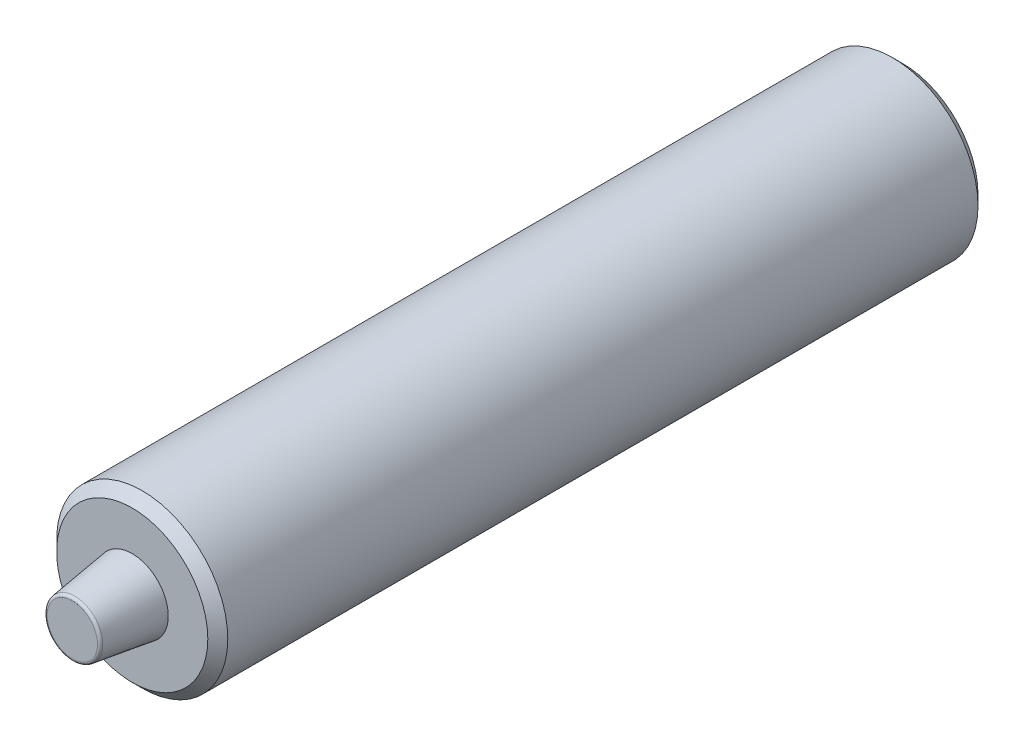
from build123d import *

# Parameters (mm, degrees)
CUT_EXTRUDE1_DEPTH = 5
SKETCH5_W          = 12
SKETCH5_H          = 4
CUT_EXTRUDE2_DEPTH = 3


with BuildPart() as part:
    # Sketch1 → Revolve1 (revolve)
    with BuildSketch(Plane(origin=(0, 0, 0), x_dir=(0, 0, -1), z_dir=(1, 0, 0)), mode=Mode.PRIVATE) as revolve1_sk:
        Polygon((0, 0), (0, 5.3), (0.7, 6), (53.3, 6), (54, 5.3), (54, 0), align=None)
    revolve(revolve1_sk.sketch.rotate(Axis((0, 0, -54), (0, 0, 1)), 270), axis=Axis((0, 0, -54), (0, 0, 1)))

    # Sketch2 → Cut-Revolve1 (revolve, cut)
    with BuildSketch(Plane(origin=(0, 0, 0), x_dir=(0, 0, -1), z_dir=(1, 0, 0)), mode=Mode.PRIVATE) as cut_revolve1_sk:
        Polygon((37, 0), (37, 3.4585), (49, 3.4585), (49, 4), (53.2, 4), (54, 4.8), (54, 0), align=None)
    revolve(cut_revolve1_sk.sketch.rotate(Axis((0, 0, -54), (0, 0, 1)), 270), axis=Axis((0, 0, -54), (0, 0, 1)), mode=Mode.SUBTRACT)

    # Sketch3 → Revolve2 (revolve)
    with BuildSketch(Plane(origin=(0, 0, 0), x_dir=(0, 0, -1), z_dir=(1, 0, 0)), mode=Mode.PRIVATE) as revolve2_sk:
        with BuildLine():
            Line((-4.2, 0), (-4.2, 1.762627227))
            ThreePointArc((-4.2, 1.762627227), (-4.150941916, 1.893839033), (-4.02783462, 1.960680841))
            Line((-4.02783462, 1.960680841), (2.3, 2.85))
            Line((2.3, 2.85), (2.3, 0))
            Line((2.3, 0), (-4.2, 0))
        make_face()
    revolve(revolve2_sk.sketch.rotate(Axis((0, 0, -2.3), (0, 0, 1)), 90), axis=Axis((0, 0, -2.3), (0, 0, 1)))

    # Sketch4 → Cut-Extrude1 (cut)
    with BuildSketch(Plane.XY.offset(-54)):
        Polygon((-4, -2.309401077), (0, -4.618802154), (4, -2.309401077), (4, 2.309401077), (0, 4.618802154), (-4, 2.309401077), align=None)
    extrude(amount=CUT_EXTRUDE1_DEPTH, mode=Mode.SUBTRACT)

    # Sketch5 → Revolve3 (revolve)
    with BuildSketch(Plane(origin=(0, 0, 0), x_dir=(0, 0, -1), z_dir=(1, 0, 0)), mode=Mode.PRIVATE) as revolve3_sk:
        with Locations((39, 2)):
            Rectangle(SKETCH5_W, SKETCH5_H)
    revolve(revolve3_sk.sketch.rotate(Axis((0, 0, -45), (0, 0, 1)), 270), axis=Axis((0, 0, -45), (0, 0, 1)))

    # Sketch6 → Cut-Extrude2 (cut)
    with BuildSketch(Plane.XY.offset(-45)):
        Polygon((-2, -1.154700538), (0, -2.309401077), (2, -1.154700538), (2, 1.154700538), (0, 2.309401077), (-2, 1.154700538), align=None)
    extrude(amount=CUT_EXTRUDE2_DEPTH, mode=Mode.SUBTRACT)

    # Sketch7 → Cut-Revolve2 (revolve, cut)
    with BuildSketch(Plane(origin=(0, 0, 0), x_dir=(0, 0, -1), z_dir=(1, 0, 0)), mode=Mode.PRIVATE) as cut_revolve2_sk:
        Polygon((40.845299462, 0), (42, 2), (42, 0), align=None)
    revolve(cut_revolve2_sk.sketch.rotate(Axis((0, 0, -42), (0, 0, 1)), 120.000000088), axis=Axis((0, 0, -42), (0, 0, 1)), mode=Mode.SUBTRACT)


solid = part.part
